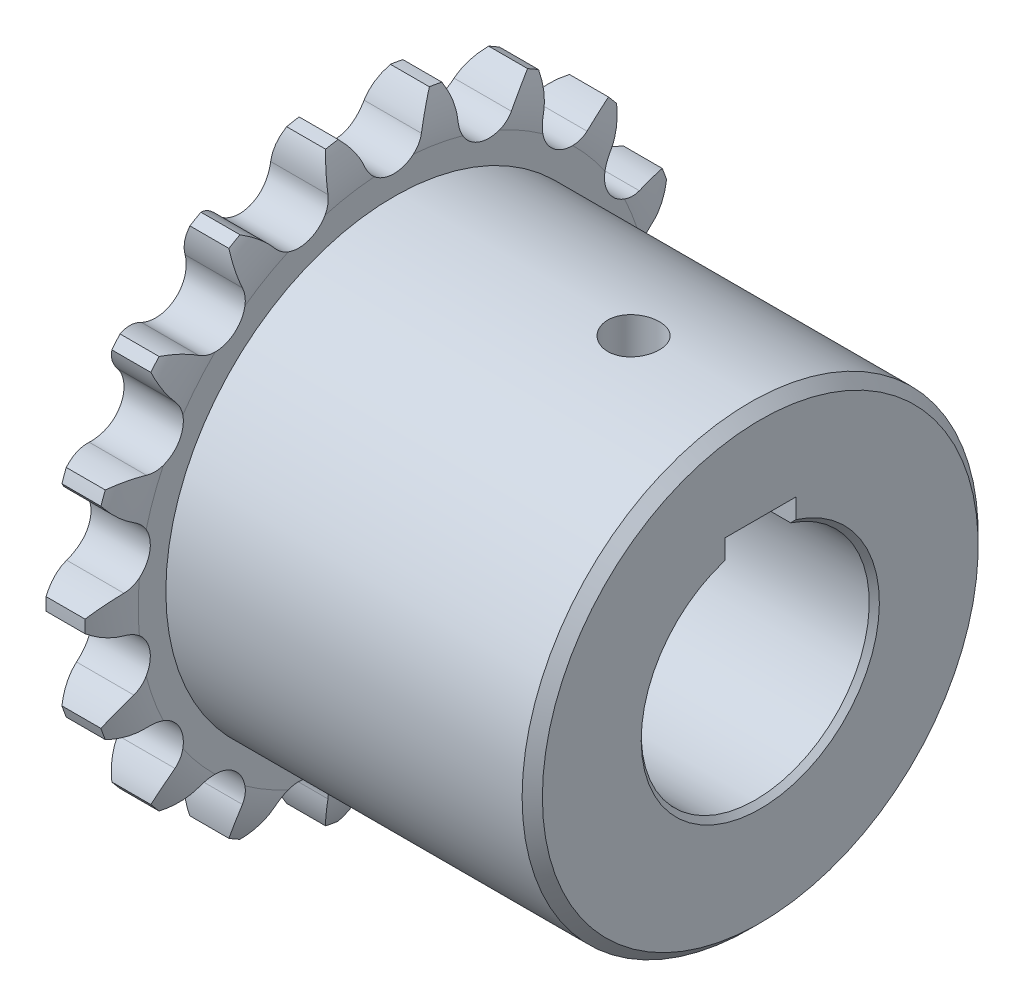
from build123d import *

# Parameters (mm, degrees)
CHAMFER1_SIZE          = 1
SKETCH8_W              = 14
SKETCH8_H              = 10.436828336
CUT_EXTRUDE2_DEPTH     = 107
CUT_EXTRUDE3_DEPTH     = 107
CIRPATTERN1_COUNT      = 18
M12_TAPPED_HOLE1_D     = 10.2
M12_TAPPED_HOLE1_DEPTH = 42.75
M12_TAPPED_HOLE1_TIP   = 3.064389157


with BuildPart() as part:
    # Sketch1 → Revolve1 (revolve)
    with BuildSketch(Plane.XY, mode=Mode.PRIVATE) as revolve1_sk:
        with BuildLine():
            Line((0, -22.5), (84, -22.5))
            Line((84, -22.5), (84, -43))
            Line((84, -43), (82, -45))
            Line((82, -45), (11.7, -45))
            Line((11.7, -45), (11.7, -50.464718626))
            ThreePointArc((11.7, -50.464718626), (11.193242009, -54.823617569), (9.7, -58.95))
            Line((9.7, -58.95), (2, -58.95))
            ThreePointArc((2, -58.95), (0.506757991, -54.823617569), (0, -50.464718626))
            Line((0, -50.464718626), (0, -22.5))
        make_face()
    revolve(revolve1_sk.sketch.rotate(Axis((0, 0, 0), (1, 0, 0)), 270), axis=Axis((0, 0, 0), (1, 0, 0)))

    # Chamfer1
    chamfer1_edges = [part.edges().sort_by_distance(p)[0] for p in [
        (0, 0, -22.5),
        (84, 0, -22.5),
    ]]
    chamfer(chamfer1_edges, length=CHAMFER1_SIZE)

    # Sketch8 → Cut-Extrude2 (cut)
    with BuildSketch(Plane(origin=(84, 0, 0), x_dir=(0, 0, -1), z_dir=(1, 0, 0))):
        with Locations((0, 21.081585832)):
            Rectangle(SKETCH8_W, SKETCH8_H)
    extrude(amount=-CUT_EXTRUDE2_DEPTH, mode=Mode.SUBTRACT)

    # Sketch7 → Cut-Extrude3 (cut)
    with BuildSketch(Plane.ZY):
        with BuildLine():
            ThreePointArc((-5.625785764, 52.902422335), (0, 48.9), (5.625785764, 52.902422335))
            ThreePointArc((5.625785764, 52.902422335), (7.006150906, 55.77389984), (9, 58.258926355))
            ThreePointArc((9, 58.258926355), (0, 58.95), (-9, 58.258926355))
            ThreePointArc((-9, 58.258926355), (-7.006150906, 55.77389984), (-5.625785764, 52.902422335))
        make_face()
    cut_extrude3 = extrude(amount=-CUT_EXTRUDE3_DEPTH, mode=Mode.SUBTRACT)

    # CirPattern1: Cut-Extrude3 ×18 about axis
    cirpattern1_axis = Axis((0, 0, 0), (1, 0, 0))
    for i in range(1, CIRPATTERN1_COUNT):
        add(cut_extrude3.rotate(cirpattern1_axis, i * 360 / CIRPATTERN1_COUNT), mode=Mode.SUBTRACT)

    # M12 Tapped Hole1
    with Locations(Plane(origin=(0, 26.3, 0), x_dir=(-1, 0, 0), z_dir=(0, -1, 0))):
        with Locations((-59, 0)):
            Hole(M12_TAPPED_HOLE1_D / 2, depth=M12_TAPPED_HOLE1_DEPTH)
            with Locations((0, 0, -(M12_TAPPED_HOLE1_DEPTH + M12_TAPPED_HOLE1_TIP / 2))):  # 118° drill point
                Cone(0, M12_TAPPED_HOLE1_D / 2, M12_TAPPED_HOLE1_TIP, mode=Mode.SUBTRACT)


solid = part.part
